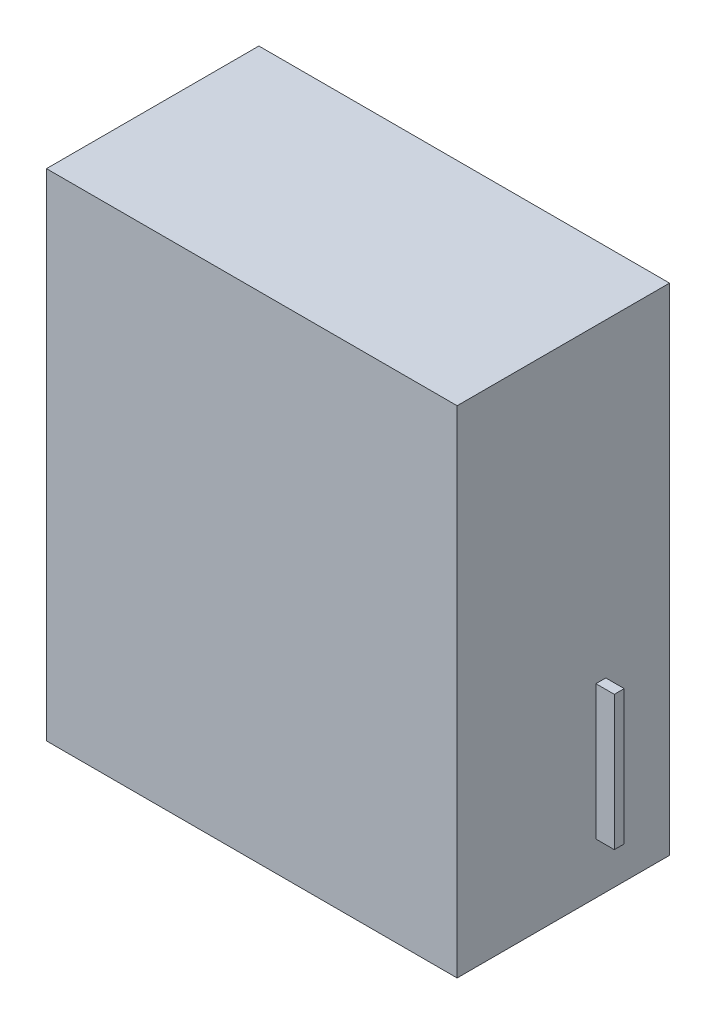
from build123d import *

# Parameters (mm, degrees)
SKETCH_1_W          = 290
SKETCH_1_H          = 150
EXTRUDE_1_DEPTH     = 350
SKETCH_2_R          = 7
EXTRUDE_2_DEPTH     = 5
SKETCH_3_W          = 145
SKETCH_3_H          = 23
CUT_EXTRUDE_1_DEPTH = 1
SKETCH_4_W          = 20
SKETCH_4_H          = 15
EXTRUDE_3_DEPTH     = 1.5
EXTRUDE_4_DEPTH     = 4.5
SKETCH_6_W          = 7
SKETCH_6_H          = 95
EXTRUDE_5_DEPTH     = 13


with BuildPart() as part:
    # 草图1 → 凸台-拉伸1 (new body)
    with BuildSketch(Plane(origin=(0, 0, 0), x_dir=(1, 0, 0), z_dir=(0, 1, 0))):
        Rectangle(SKETCH_1_W, SKETCH_1_H)
    extrude(amount=EXTRUDE_1_DEPTH)

    # 草图2 → 凸台-拉伸2 (add)
    with BuildSketch(Plane.XZ):
        with Locations(Location((-110, 63, 0), (0, 0, 90))):
            Circle(SKETCH_2_R)
        with Locations(Location((110, 63, 0), (0, 0, 90))):
            Circle(SKETCH_2_R)
        with Locations(Location((110, -67, 0), (0, 0, 90))):
            Circle(SKETCH_2_R)
        with Locations(Location((-110, -67, 0), (0, 0, 90))):
            Circle(SKETCH_2_R)
    extrude(amount=EXTRUDE_2_DEPTH)

    # 草图3 → 切除-拉伸1 (cut)
    with BuildSketch(Plane.ZY.offset(145)):
        with Locations((0, 160.5)):
            Rectangle(SKETCH_3_W, SKETCH_3_H)
    extrude(amount=-CUT_EXTRUDE_1_DEPTH, mode=Mode.SUBTRACT)

    # 草图4 → 凸台-拉伸3 (add)
    with BuildSketch(Plane.ZY.offset(144)):
        with Locations((-56.5, 160.5)):
            Rectangle(SKETCH_4_W, SKETCH_4_H)
    extrude(amount=EXTRUDE_3_DEPTH)

    # 草图5 → 凸台-拉伸4 (add, symmetric)
    with BuildSketch(Plane(origin=(0, 160.5, 0), x_dir=(-1, 0, 0), z_dir=(0, -1, 0))):
        with BuildLine():
            Line((145.5, 63.5), (149.5, 60.5))
            ThreePointArc((149.5, 60.5), (146.755035208, 55.270896288), (145.5, 49.5))
            Line((145.5, 49.5), (145.5, 63.5))
        make_face()
    extrude(amount=EXTRUDE_4_DEPTH, both=True)

    # 草图6 → 凸台-拉伸5 (add)
    with BuildSketch(Plane(origin=(145, 0, 0), x_dir=(0, 0, -1), z_dir=(1, 0, 0))):
        with Locations((26.5, 83.5)):
            Rectangle(SKETCH_6_W, SKETCH_6_H)
    extrude(amount=EXTRUDE_5_DEPTH)


solid = part.part
